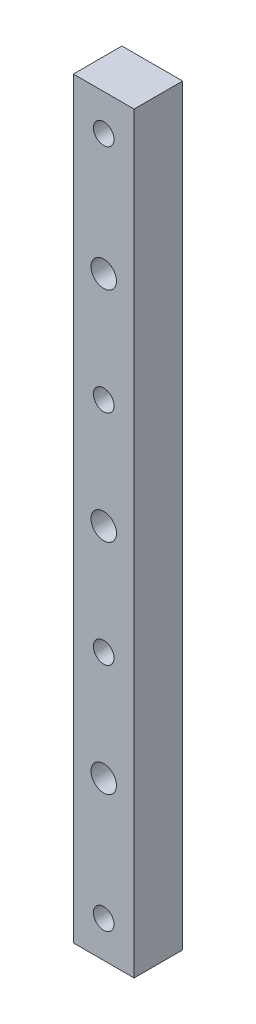
from build123d import *

# Parameters (mm, degrees)
SKETCH1_W                   = 25
SKETCH1_H                   = 310
BOSS_EXTRUDE1_DEPTH         = 20
SKETCH3_R                   = 4.25
CUT_EXTRUDE1_DEPTH          = 30
SKETCH5_R                   = 6.5
CUT_EXTRUDE3_DEPTH          = 10
M12X1_25_TAPPED_HOLE1_D     = 10.5
M12X1_25_TAPPED_HOLE1_DEPTH = 30.25
M12X1_25_TAPPED_HOLE1_TIP   = 3.15451825


with BuildPart() as part:
    # Sketch1 → Boss-Extrude1 (new body)
    with BuildSketch(Plane.XY):
        Rectangle(SKETCH1_W, SKETCH1_H)
    extrude(amount=BOSS_EXTRUDE1_DEPTH)

    # Sketch3 → Cut-Extrude1 (cut)
    with BuildSketch(Plane.XY.offset(20)):
        with Locations((0, 140)):
            Circle(SKETCH3_R)
        with Locations((0, 45)):
            Circle(SKETCH3_R)
        with Locations((0, -45)):
            Circle(SKETCH3_R)
        with Locations((0, -140)):
            Circle(SKETCH3_R)
    extrude(amount=-CUT_EXTRUDE1_DEPTH, mode=Mode.SUBTRACT)

    # Sketch5 → Cut-Extrude3 (cut)
    with BuildSketch(Plane(origin=(0, 0, 0), x_dir=(-1, 0, 0), z_dir=(0, 0, -1))):
        with Locations((0, 140)):
            Circle(SKETCH5_R)
        with Locations((0, 45)):
            Circle(SKETCH5_R)
        with Locations((0, -45)):
            Circle(SKETCH5_R)
        with Locations((0, -140)):
            Circle(SKETCH5_R)
    extrude(amount=-CUT_EXTRUDE3_DEPTH, mode=Mode.SUBTRACT)

    # M12x1.25 Tapped Hole1
    with Locations(Plane(origin=(0, 0, 0), x_dir=(-1, 0, 0), z_dir=(0, 0, -1))):
        with Locations((0, 90), (0, 0), (0, -90)):
            Hole(M12X1_25_TAPPED_HOLE1_D / 2, depth=M12X1_25_TAPPED_HOLE1_DEPTH)
            with Locations((0, 0, -(M12X1_25_TAPPED_HOLE1_DEPTH + M12X1_25_TAPPED_HOLE1_TIP / 2))):  # 118° drill point
                Cone(0, M12X1_25_TAPPED_HOLE1_D / 2, M12X1_25_TAPPED_HOLE1_TIP, mode=Mode.SUBTRACT)


solid = part.part
